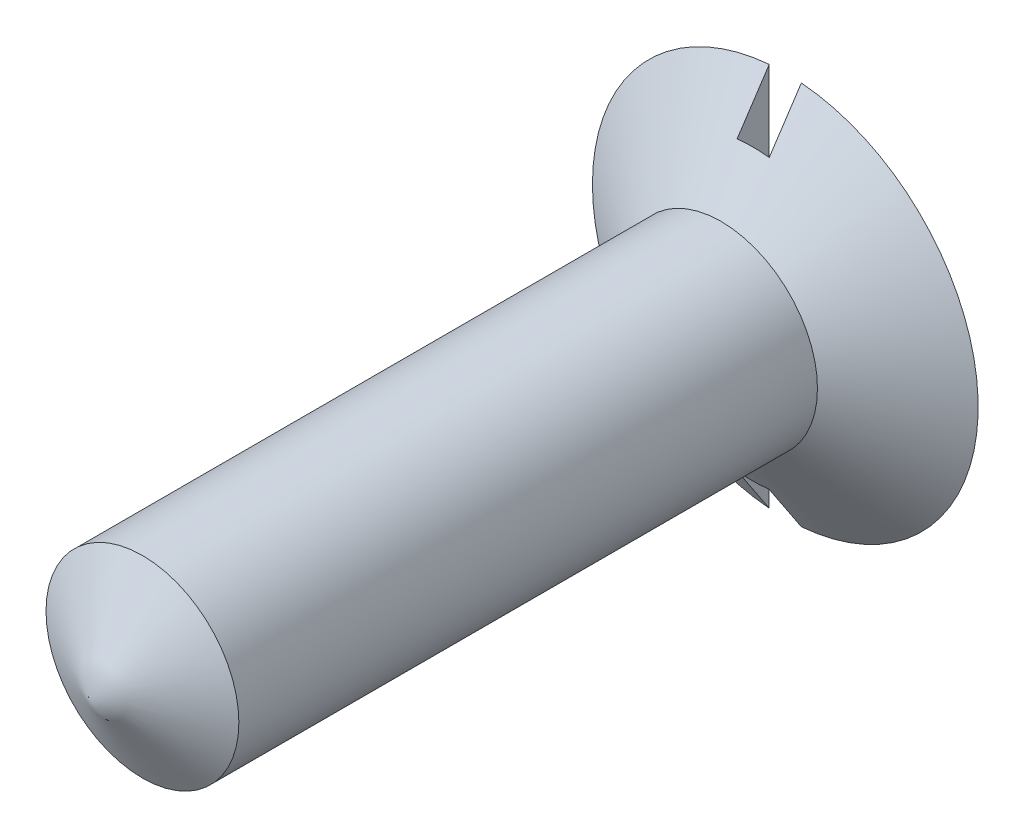
SolidWorks part; units mm, degrees
material "Silicon"
ref_plane "Front Plane" through (0, 0, 0) normal (0, 0, 1) x (1, 0, 0)
ref_plane "Top Plane" through (0, 0, 0) normal (0, 1, 0) x (1, 0, 0)
ref_plane "Right Plane" through (0, 0, 0) normal (1, 0, 0) x (0, 0, -1)
sketch "Sketch1" plane through (0, 0, 0) normal (0, 1, 0) x (1, 0, 0)
  line L0 (0, 16.5) -> (0, 13.5)
  line L1 (0, 13.5) -> (0, -13.5)
  line L2 (0, -13.5) -> (0, -16)
  line L5 (0, 16.5) -> (9, 16.5)
  line L6 (4.5, 13.5) -> (4.5, -13.5)
  line L7 (4.5, -13.5) -> (0, -16)
  line L8 (0, 13.5) -> (4.5, 13.5)
  line L9 (0, -13.5) -> (4.5, -13.5)
  line L10 (9, 16.5) -> (4.5, 13.5)
  dimension "D1" = 3
  dimension "D2" = 27
  dimension "D3" = 2.5
  dimension "D5" = 9
  dimension "D6" = 4.5
revolve "Revolve3" add sketch "Sketch1" angle 360 about L1
sketch "Sketch2" plane through (0, 0, 0) normal (0, 1, 0) x (1, 0, 0)
  line L0 (0, 16.5) -> (0.75, 16.5)
  line L1 (9, 16.5) -> (-9, 16.5) construction
  line L2 (0.75, 16.5) -> (0.75, 15)
  line L3 (-0.75, 15) -> (0.75, 15)
  line L5 (-0.75, 15) -> (-0.75, 16.5)
  line L6 (-0.75, 16.5) -> (0, 16.5)
  dimension "D1" = 0.75
  dimension "D2" = 0.75
  dimension "D3" = 1.5
extrude "Cut-Extrude1" cut sketch "Sketch2" against normal mid plane 30
